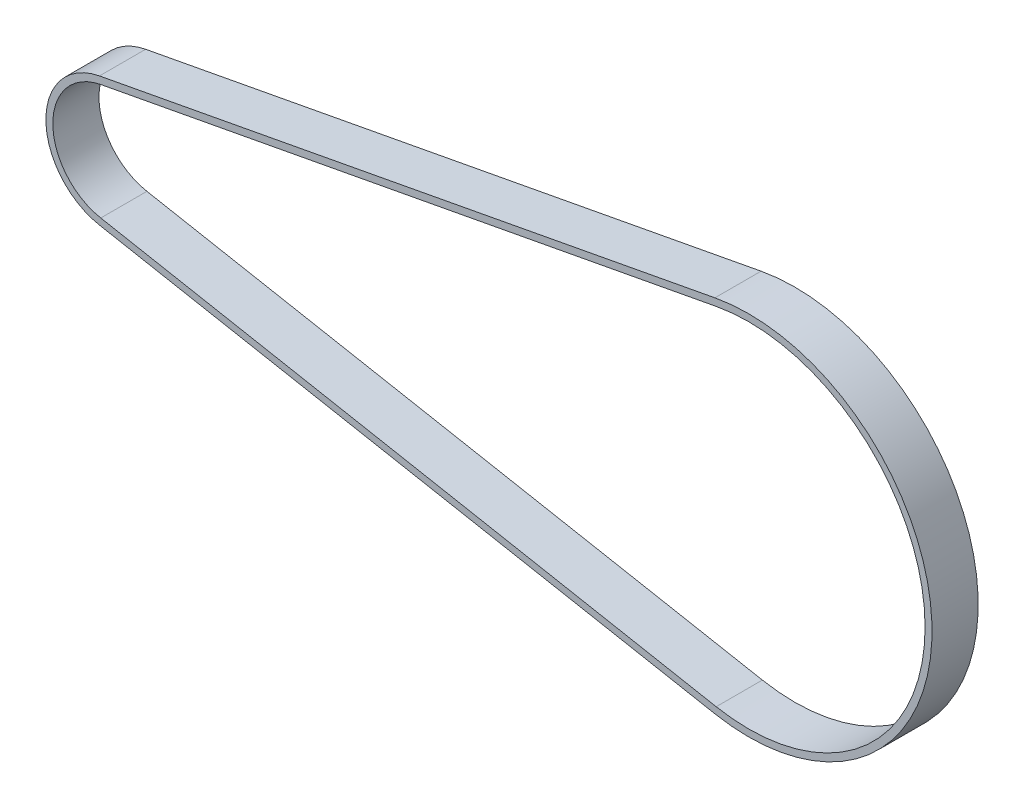
from build123d import *

# Parameters (mm, degrees)
BOSS_EXTRUDE1_DEPTH = 4


with BuildPart() as part:
    # Sketch1 → Boss-Extrude1 (new body)
    with BuildSketch(Plane.XY):
        with BuildLine():
            Line((-1.050789402, -5.597219545), (52.269967391, -15.607347914))
            ThreePointArc((52.269967391, -15.607347914), (71.08, 0), (52.269967391, 15.607347914))
            Line((52.269967391, 15.607347914), (-1.050789402, 5.597219545))
            ThreePointArc((-1.050789402, 5.597219545), (-5.695, 0), (-1.050789402, -5.597219545))
        make_face()
        with BuildLine():
            Line((-0.94008288, 5.007521261), (52.380673913, 15.01764963))
            ThreePointArc((52.380673913, 15.01764963), (70.48, 0), (52.380673913, -15.01764963))
            Line((52.380673913, -15.01764963), (-0.94008288, -5.007521261))
            ThreePointArc((-0.94008288, -5.007521261), (-5.095, 0), (-0.94008288, 5.007521261))
        make_face(mode=Mode.SUBTRACT)
    extrude(amount=BOSS_EXTRUDE1_DEPTH)


solid = part.part
